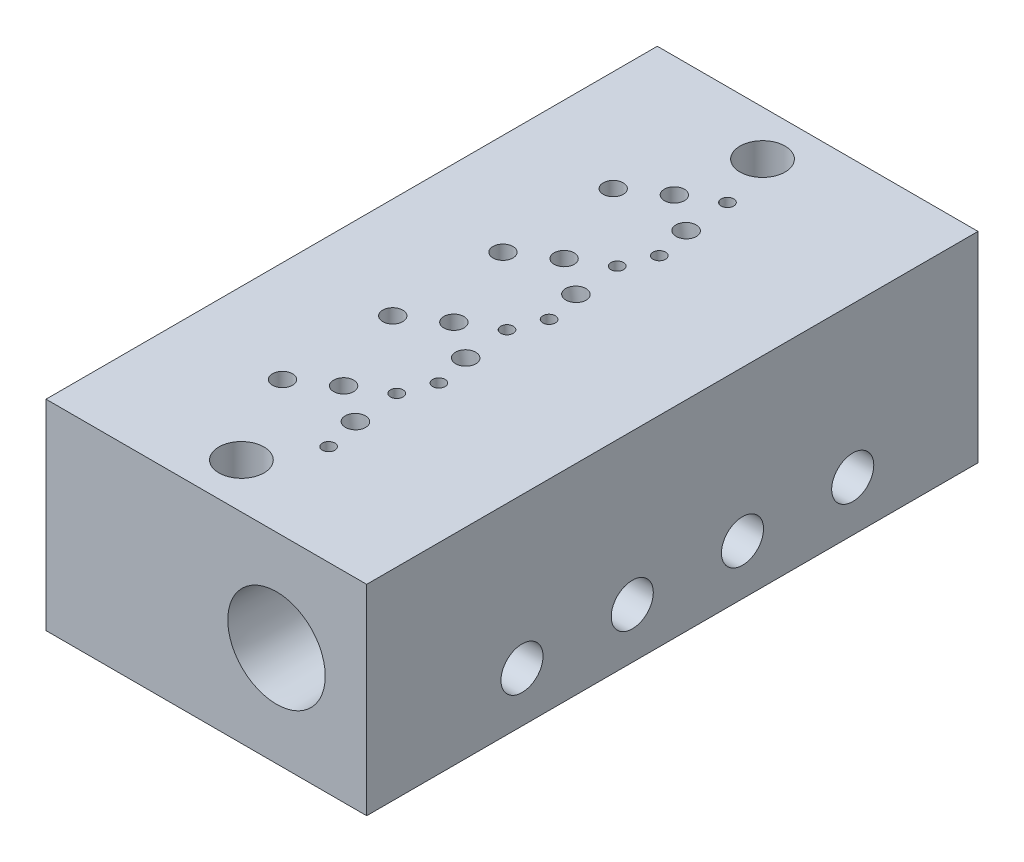
from build123d import *

# Parameters (mm, degrees)
SKETCH1_W                    = 32
SKETCH1_H                    = 20
BOSS_EXTRUDE1_DEPTH          = 61
SKETCH8_R                    = 2.25
CUT_EXTRUDE3_DEPTH           = 53
SKETCH9_R                    = 1
CUT_EXTRUDE4_DEPTH           = 10
CUT_EXTRUDE5_REACH           = 72.509
SKETCH16_R                   = 1
SKETCH17_R                   = 1
CUT_EXTRUDE6_DEPTH           = 15
M1_6_TAPPED_HOLE1_AT_2_COUNT = 2
M1_6_TAPPED_HOLE1_AT_2_PITCH = 8.089499366
F_4_5_4_5_DIAMETER_HOLE1_D   = 4.5
LPATTERN1_COUNT              = 4
LPATTERN1_PITCH              = 11


with BuildPart() as part:
    # Sketch1 → Boss-Extrude1 (new body)
    with BuildSketch(Plane.XY):
        with Locations((-16, -10)):
            Rectangle(SKETCH1_W, SKETCH1_H)
    extrude(amount=-BOSS_EXTRUDE1_DEPTH)

    # Sketch5 → 1/8 Rc Tapped Hole2 (revolve, cut)
    with BuildSketch(Plane(origin=(-9, -10, 0), x_dir=(0, -1, 0), z_dir=(1, 0, 0))):
        Polygon((0, 0), (0, 10.873399445), (3.95, 8.5), (3.95, 7.4), (4.632997004, 7.4), (4.864, 0), align=None)
    revolve(axis=Axis((-9, -10, 6.35), (0, 0, -1)), mode=Mode.SUBTRACT)

    # Sketch8 → Cut-Extrude3 (cut)
    with BuildSketch(Plane.XY):
        with Locations(Location((-10.5, -10, 0), (0, 0, 7.55e-07))):
            Circle(SKETCH8_R)
    extrude(amount=-CUT_EXTRUDE3_DEPTH, mode=Mode.SUBTRACT)

    # Sketch9 → Cut-Extrude4 (cut)
    with BuildSketch(Plane(origin=(0, 0, 0), x_dir=(1, 0, 0), z_dir=(0, 1, 0))):
        with Locations(Location((-21.9, 13.5, 0), (0, 0, 270))):
            Circle(SKETCH9_R)
    cut_extrude4 = extrude(amount=-CUT_EXTRUDE4_DEPTH, mode=Mode.SUBTRACT)

    # Sketch13 → M5 Tapped Hole2 (revolve, cut)
    with BuildSketch(Plane(origin=(0, -15, -15.5), x_dir=(0, 0, -1), z_dir=(0, 1, 0))):
        Polygon((0, 0), (0, 21.2618073), (2.1, 20), (2.1, 0), align=None)
    m5_tapped_hole2 = revolve(axis=Axis((6.35, -15, -15.5), (-1, 0, 0)), mode=Mode.SUBTRACT)

    # Cut-Extrude5: up to this plane
    cut_extrude5_end = Plane(origin=(-32, 0, -61), z_dir=(0, 1, 0))
    # Sketch16 → Cut-Extrude5 (cut, up to the surface)
    with BuildSketch(Plane(origin=(1.562833599, -8.863269777, 0), x_dir=(0.984807753012208, 0.17364817766693072, 0), z_dir=(-0.17364817766693072, 0.984807753012208, 0)), mode=Mode.PRIVATE) as cut_extrude5_sk1:
        with Locations((-14.4, 13.5)):
            Circle(SKETCH16_R)
    cut_extrude5_tool1 = split(extrude(cut_extrude5_sk1.sketch, amount=CUT_EXTRUDE5_REACH, mode=Mode.PRIVATE), bisect_by=cut_extrude5_end, keep=Keep.BOTH, mode=Mode.PRIVATE)
    cut_extrude5 = cut_extrude5_tool1.solids().sort_by_distance((-12.618398, -11.363804, -13.5))[0]
    add(cut_extrude5, mode=Mode.SUBTRACT)

    # Sketch17 → Cut-Extrude6 (cut)
    with BuildSketch(Plane(origin=(0, 0, 0), x_dir=(1, 0, 0), z_dir=(0, 1, 0))):
        with Locations(Location((-18.3, 16, 0), (0, 0, 270))):
            Circle(SKETCH17_R)
    cut_extrude6 = extrude(amount=-CUT_EXTRUDE6_DEPTH, mode=Mode.SUBTRACT)

    # Sketch19 → M1.6 Tapped Hole1 (revolve, cut)
    with BuildSketch(Plane(origin=(-13.8, 0, -10), x_dir=(0, 0, 1), z_dir=(1, 0, 0))):
        Polygon((0, 0), (0, 4.625537887), (0.625, 4.25), (0.625, 0), align=None)
    m1_6_tapped_hole1 = revolve(axis=Axis((-13.8, 6.35, -10), (0, -1, 0)), mode=Mode.SUBTRACT)

    # M1.6 Tapped Hole1 at 2: M1.6 Tapped Hole1 ×2
    with Locations(*[Vector(-0.14834045293024456, 0, -0.9889363528682976) * (i * M1_6_TAPPED_HOLE1_AT_2_PITCH) for i in range(1, M1_6_TAPPED_HOLE1_AT_2_COUNT)]):
        add(m1_6_tapped_hole1, mode=Mode.SUBTRACT)

    # Ø4.5 (4.5) Diameter Hole1 (through all)
    with Locations(Plane(origin=(0, 0, 0), x_dir=(1, 0, 0), z_dir=(0, 1, 0))):
        with Locations((-17, 4.5), (-17, 56.5)):
            Hole(F_4_5_4_5_DIAMETER_HOLE1_D / 2)

    # Sketch24 → Cut-Revolve1 (revolve, cut)
    with BuildSketch(Plane.XY.offset(-13.5), mode=Mode.PRIVATE) as cut_revolve1_sk:
        Polygon((-12.618398044, -11.363803536), (-11.633590291, -11.190155358), (-12.514059693, -11.955535732), align=None)
    cut_revolve1 = revolve(cut_revolve1_sk.sketch.rotate(Axis((-14.542300247, -0.452811949, -13.5), (0.17364817766693064, -0.984807753012208, 0)), 180), axis=Axis((-14.542300247, -0.452811949, -13.5), (0.17364817766693064, -0.984807753012208, 0)), mode=Mode.SUBTRACT)

    # Sketch25 → M5 Tapped Hole3 (revolve, cut)
    with BuildSketch(Plane(origin=(-32, -10, -13.5), x_dir=(0, 0, 1), z_dir=(0, 1, 0))):
        Polygon((0, 0), (0, 12.7618073), (2.1, 11.5), (2.1, 0), align=None)
    m5_tapped_hole3 = revolve(axis=Axis((-38.35, -10, -13.5), (1, 0, 0)), mode=Mode.SUBTRACT)

    # LPattern1: Cut-Extrude4, M5 Tapped Hole2, Cut-Extrude5, Cut-Extrude6, M1.6 Tapped Hole1, Cut-Revolve1, M5 Tapped Hole3 ×4
    with Locations(*[(0, 0, -i * LPATTERN1_PITCH) for i in range(1, LPATTERN1_COUNT)]):
        add(cut_extrude4, mode=Mode.SUBTRACT)
        add(m5_tapped_hole2, mode=Mode.SUBTRACT)
        add(cut_extrude5, mode=Mode.SUBTRACT)
        add(cut_extrude6, mode=Mode.SUBTRACT)
        add(m1_6_tapped_hole1, mode=Mode.SUBTRACT)
        add(cut_revolve1, mode=Mode.SUBTRACT)
        add(m5_tapped_hole3, mode=Mode.SUBTRACT)

    # LPattern1 copy 1 sketch → LPattern1 copy 1 (revolve, cut)
    with BuildSketch(Plane(origin=(-15, 0, -29), x_dir=(0, 0, 1), z_dir=(1, 0, 0))):
        Polygon((0, 0), (0, 4.625537887), (0.625, 4.25), (0.625, 0), align=None)
    revolve(axis=Axis((-15, 6.35, -29), (0, -1, 0)), mode=Mode.SUBTRACT)

    # LPattern1 copy 2 sketch → LPattern1 copy 2 (revolve, cut)
    with BuildSketch(Plane(origin=(-15, 0, -40), x_dir=(0, 0, 1), z_dir=(1, 0, 0))):
        Polygon((0, 0), (0, 4.625537887), (0.625, 4.25), (0.625, 0), align=None)
    revolve(axis=Axis((-15, 6.35, -40), (0, -1, 0)), mode=Mode.SUBTRACT)

    # LPattern1 copy 3 sketch → LPattern1 copy 3 (revolve, cut)
    with BuildSketch(Plane(origin=(-15, 0, -51), x_dir=(0, 0, 1), z_dir=(1, 0, 0))):
        Polygon((0, 0), (0, 4.625537887), (0.625, 4.25), (0.625, 0), align=None)
    revolve(axis=Axis((-15, 6.35, -51), (0, -1, 0)), mode=Mode.SUBTRACT)


solid = part.part
